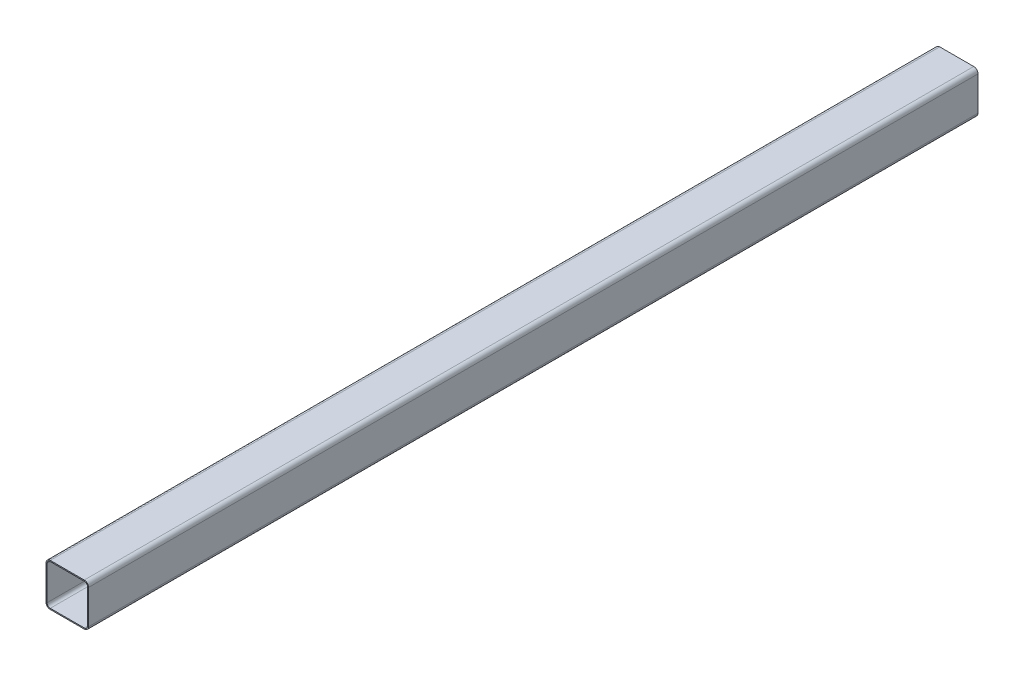
from build123d import *

# Parameters (mm, degrees)
BOSS_EXTRUDE1_DEPTH = 4180


with BuildPart() as part:
    # Sketch1 → Boss-Extrude1 (new body)
    with BuildSketch(Plane.XY):
        with BuildLine():
            Line((-80, 100), (80, 100))
            ThreePointArc((80, 100), (94.142135624, 94.142135624), (100, 80))
            Line((100, 80), (100, -80))
            ThreePointArc((100, -80), (94.142135624, -94.142135624), (80, -100))
            Line((80, -100), (-80, -100))
            ThreePointArc((-80, -100), (-94.142135624, -94.142135624), (-100, -80))
            Line((-100, -80), (-100, 80))
            ThreePointArc((-100, 80), (-94.142135624, 94.142135624), (-80, 100))
        make_face()
        with BuildLine():
            Line((-95, 80), (-95, -80))
            ThreePointArc((-95, -80), (-90.606601718, -90.606601718), (-80, -95))
            Line((-80, -95), (80, -95))
            ThreePointArc((80, -95), (90.606601718, -90.606601718), (95, -80))
            Line((95, -80), (95, 80))
            ThreePointArc((95, 80), (90.606601718, 90.606601718), (80, 95))
            Line((80, 95), (-80, 95))
            ThreePointArc((-80, 95), (-90.606601718, 90.606601718), (-95, 80))
        make_face(mode=Mode.SUBTRACT)
    extrude(amount=BOSS_EXTRUDE1_DEPTH)


solid = part.part
